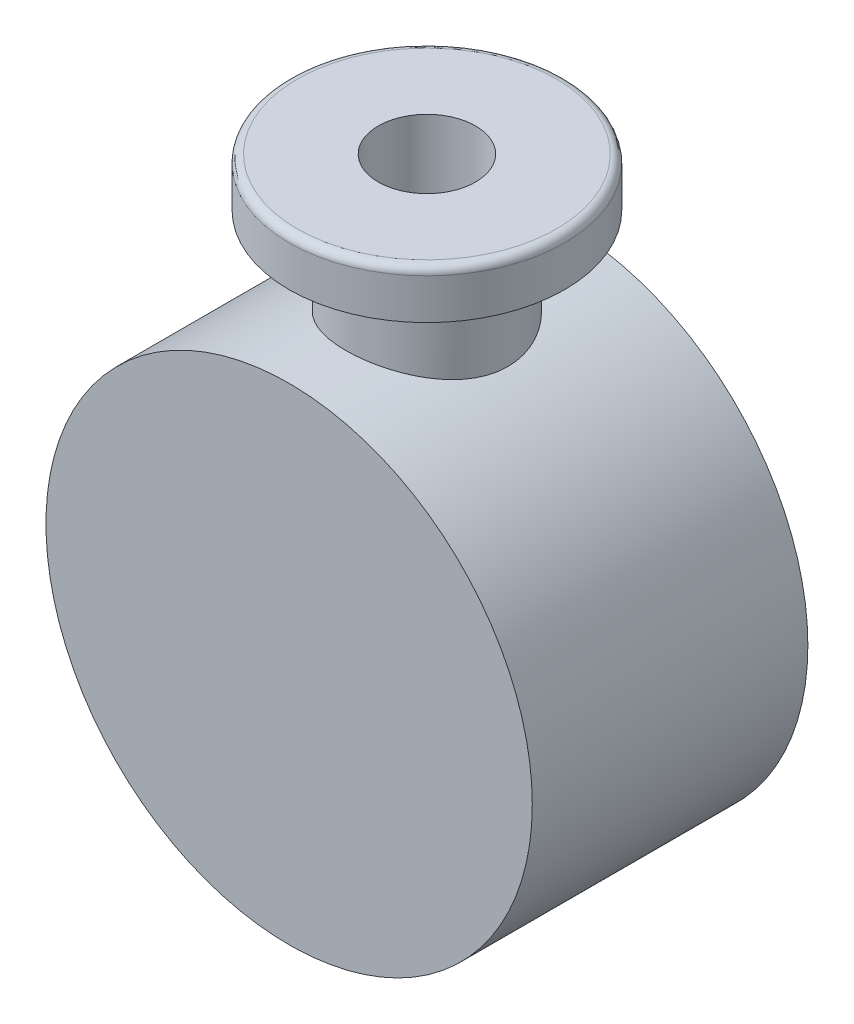
SolidWorks part; units mm, degrees
ref_plane "Front Plane" through (0, 0, 0) normal (0, 0, 1) x (1, 0, 0)
ref_plane "Top Plane" through (0, 0, 0) normal (0, 1, 0) x (1, 0, 0)
ref_plane "Right Plane" through (0, 0, 0) normal (1, 0, 0) x (0, 0, -1)
other "Configuration Table"
sketch "Sketch1" plane through (0, 0, 0) normal (0, 0, 1) x (1, 0, 0)
  circle A0 centre (0, 0) radius 15
  dimension "D1" = 30
extrude "Boss-Extrude1" add sketch "Sketch1" along normal mid plane 17
sketch "Sketch2" plane through (0, 0, 0) normal (0, 1, 0) x (1, 0, 0)
  circle A0 centre (0, 0) radius 3
  dimension "D1" = 6
extrude "Cut-Extrude1" cut sketch "Sketch2" against normal through all both and the other way through all
ref_plane "Plane1" through (0, 20, 0) normal (0, 1, 0) x (1, 0, 0)
sketch "Sketch3" plane through (0, 20, 0) normal (0, 1, 0) x (1, 0, 0)
  circle A0 centre (0, 0) radius 5
  circle A1 centre (0, 0) radius 3 construction
  circle A2 centre (0, 0) radius 3
  dimension "D1" = 10
extrude "Boss-Extrude2" add sketch "Sketch3" against normal up to surface (5 mm away)
sketch "Sketch4" plane through (0, 20, 0) normal (0, 1, 0) x (1, 0, 0)
  circle A0 centre (0, 0) radius 8.5
  circle A1 centre (0, 0) radius 3 construction
  circle A2 centre (0, 0) radius 3
extrude "Boss-Extrude3" add sketch "Sketch4" along normal blind 3
fillet "Fillet1" radius 0.5 1 edges at (0, 23, 8.5)
